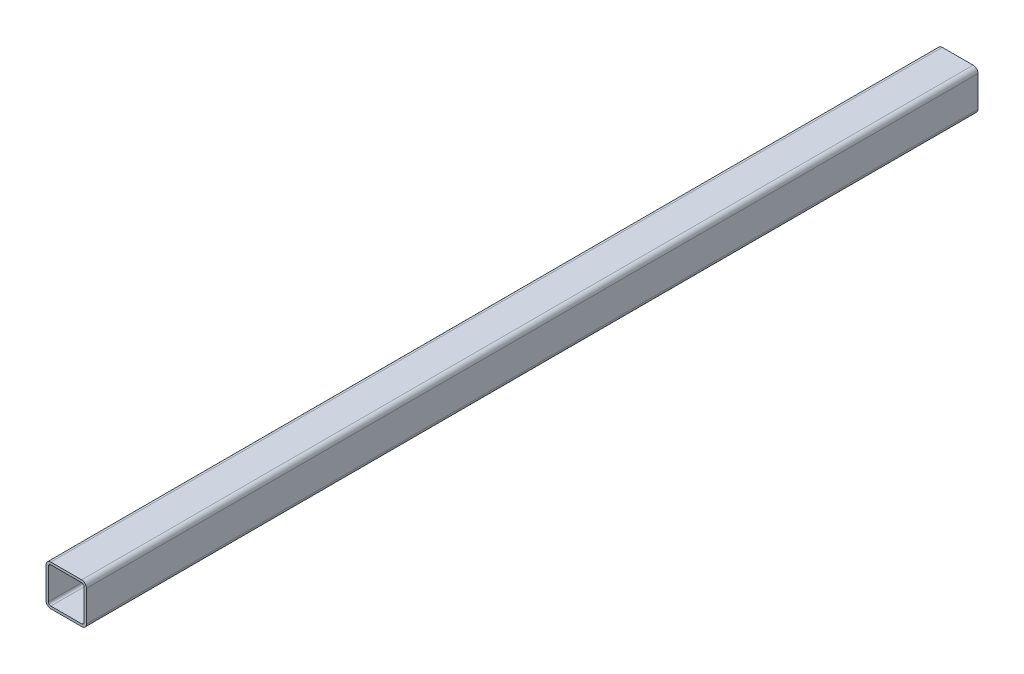
from build123d import *

# Parameters (mm, degrees)
GB_6728_1986_050_X_50_X_3_1_DEPTH = 1100
HOLE_WIZARD_M6_1_D                = 5
HOLE_WIZARD_M6_1_DEPTH            = 15
HOLE_WIZARD_M6_1_TIP              = 1.502151548


with BuildPart() as part:
    # Sketch1 → Gb／6728-1986方形空心型钢 050 X 50 X 3(1) (new body)
    with BuildSketch(Plane(origin=(0, 0, 0), x_dir=(-1, 0, 0), z_dir=(0, 0, -1))):
        with BuildLine():
            Line((-19, -25), (19, -25))
            ThreePointArc((19, -25), (23.242640687, -23.242640687), (25, -19))
            Line((25, -19), (25, 19))
            ThreePointArc((25, 19), (23.242640687, 23.242640687), (19, 25))
            Line((19, 25), (-19, 25))
            ThreePointArc((-19, 25), (-23.242640687, 23.242640687), (-25, 19))
            Line((-25, 19), (-25, -19))
            ThreePointArc((-25, -19), (-23.242640687, -23.242640687), (-19, -25))
        make_face()
        with BuildLine():
            Line((-19, -22), (19, -22))
            ThreePointArc((19, -22), (21.121320344, -21.121320344), (22, -19))
            Line((22, -19), (22, 19))
            ThreePointArc((22, 19), (21.121320344, 21.121320344), (19, 22))
            Line((19, 22), (-19, 22))
            ThreePointArc((-19, 22), (-21.121320344, 21.121320344), (-22, 19))
            Line((-22, 19), (-22, -19))
            ThreePointArc((-22, -19), (-21.121320344, -21.121320344), (-19, -22))
        make_face(mode=Mode.SUBTRACT)
    extrude(amount=GB_6728_1986_050_X_50_X_3_1_DEPTH)

    # M6 螺纹孔1
    with Locations(Plane(origin=(0, -25, 0), x_dir=(-1, 0, 0), z_dir=(0, -1, 0))):
        with Locations((-5, 100), (-5, 400), (-5, 700), (-5, 1000)):
            Hole(HOLE_WIZARD_M6_1_D / 2, depth=HOLE_WIZARD_M6_1_DEPTH)
            with Locations((0, 0, -(HOLE_WIZARD_M6_1_DEPTH + HOLE_WIZARD_M6_1_TIP / 2))):  # 118° drill point
                Cone(0, HOLE_WIZARD_M6_1_D / 2, HOLE_WIZARD_M6_1_TIP, mode=Mode.SUBTRACT)


solid = part.part
